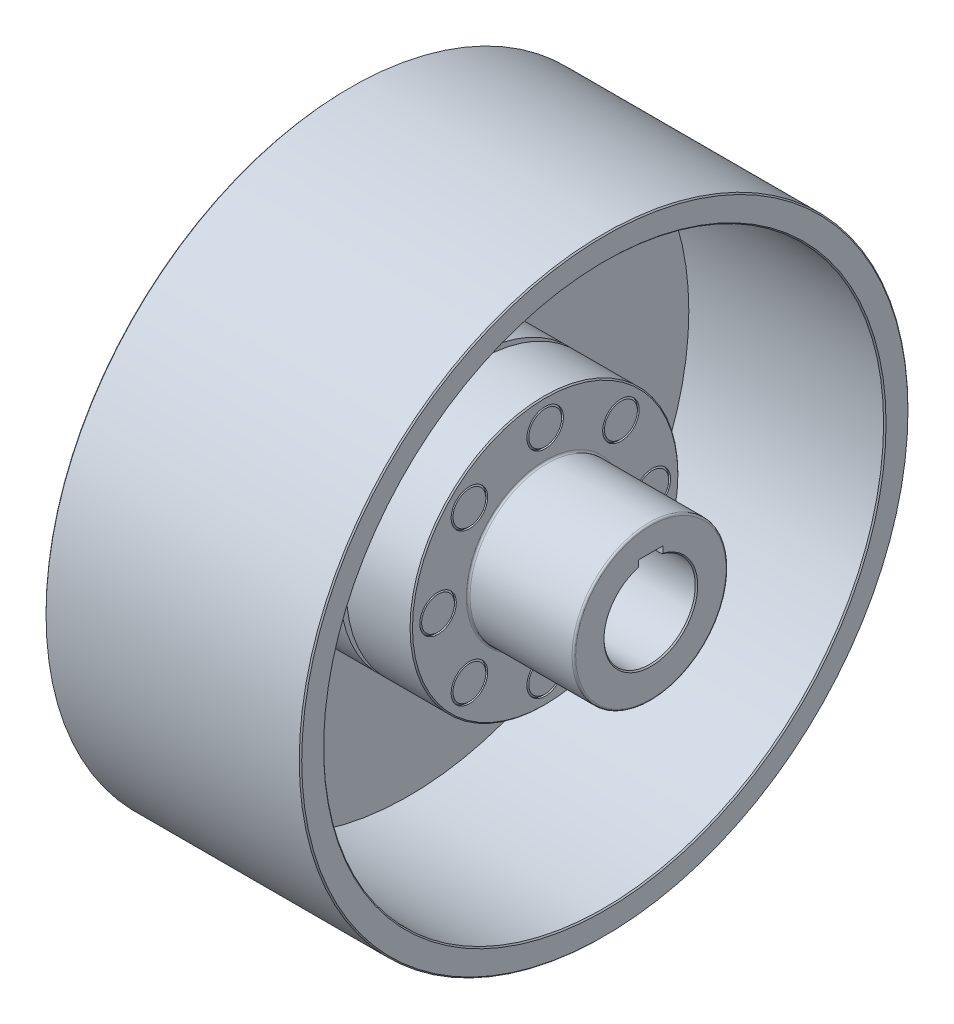
from build123d import *

# Parameters (mm, degrees)
CHAMFER1_SIZE      = 1
CHAMFER2_SIZE      = 1
CHAMFER3_SIZE      = 1
FILLET1_R          = 1.5
FILLET2_R          = 1.5
EXTRUDE1_DEPTH     = 3.375
CIRPATTERN11_COUNT = 8
SKETCH6_W          = 20
SKETCH6_H          = 9.8
CUT_EXTRUDE1_DEPTH = 455.496820734


with BuildPart() as part:
    # Sketch1 → Revolve1 (revolve)
    with BuildSketch(Plane.XY, mode=Mode.PRIVATE) as revolve1_sk:
        Polygon((-2.8, 56.925), (-30.8, 56.925), (-30.8, 37.5), (-142.8, 37.5), (-142.8, 63.25), (-61.6, 63.25), (-61.6, 68.85), (-56, 68.85), (-56, 110), (-2.8, 110), (-2.8, 104.5), (2.8, 104.5), (2.8, 110), (56, 110), (56, 63.25), (142.8, 63.25), (142.8, 37.5), (2.8, 37.5), (2.8, 0), (-2.8, 0), align=None)
    revolve(revolve1_sk.sketch.rotate(Axis((-114.849033811, 0, 0), (1, 0, 0)), 90), axis=Axis((-114.849033811, 0, 0), (1, 0, 0)))

    # Sketch2 → Revolve2 (revolve)
    with BuildSketch(Plane.XY, mode=Mode.PRIVATE) as revolve2_sk:
        Polygon((105, 250), (-105, 250), (-105, 230), (-61.6, 230), (-61.6, 68.85), (-56, 68.85), (-56, 230), (105, 230), align=None)
    revolve(revolve2_sk.sketch.rotate(Axis((0, 0, 0), (-1, 0, 0)), 90), axis=Axis((0, 0, 0), (-1, 0, 0)))

    # Sketch3 → Cut-Revolve1 (revolve, cut)
    with BuildSketch(Plane.XY, mode=Mode.PRIVATE) as cut_revolve1_sk:
        Polygon((-56, 103), (-61.6, 103), (-61.6, 88), (-56, 88), (-56, 101.5), (-54.5, 103), align=None)
        Polygon((56, 103), (54.5, 103), (56, 101.5), align=None)
    cut_revolve1 = revolve(cut_revolve1_sk.sketch.rotate(Axis((-61.6, 88, 0), (1, 0, 0)), 180), axis=Axis((-61.6, 88, 0), (1, 0, 0)), mode=Mode.SUBTRACT)

    # Chamfer1
    chamfer1_edges = [part.edges().sort_by_distance(p)[0] for p in [
        (142.8, 0, -37.5),
        (56, 0, -110),
    ]]
    chamfer(chamfer1_edges, length=CHAMFER1_SIZE)

    # Chamfer2
    chamfer2_edges = [part.edges().sort_by_distance(p)[0] for p in [
        (105, 0, 250),
        (105, 0, 230),
        (-105, 0, 230),
        (-105, 0, 250),
    ]]
    chamfer(chamfer2_edges, length=CHAMFER2_SIZE)

    # Chamfer3
    chamfer3_edges = [part.edges().sort_by_distance(p)[0] for p in [
        (-142.8, 0, -37.5),
    ]]
    chamfer(chamfer3_edges, length=CHAMFER3_SIZE)

    # Fillet1
    fillet1_edges = [part.edges().sort_by_distance(p)[0] for p in [
        (-61.6, 0, -63.25),
        (-142.8, 0, -63.25),
    ]]
    fillet(fillet1_edges, radius=FILLET1_R)

    # Fillet2
    fillet2_edges = [part.edges().sort_by_distance(p)[0] for p in [
        (142.8, 0, -63.25),
        (56, 0, -63.25),
    ]]
    fillet(fillet2_edges, radius=FILLET2_R)

    # Sketch5 → Extrude1 (add)
    with BuildSketch(Plane.ZY.offset(61.6)):
        Polygon((33.676142048, 76.971271842), (37.426142048, 79.136335352), (37.426142048, 83.46646237), (33.676142048, 85.63152588), (29.926142048, 83.46646237), (29.926142048, 79.136335352), align=None)
    extrude1 = extrude(amount=EXTRUDE1_DEPTH)

    # CirPattern11: Cut-Revolve1, Extrude1 ×8 about axis
    cirpattern11_axis = Axis((0, 0, 0), (1, 0, 0))
    add([cut_revolve1.rotate(cirpattern11_axis, i * 360 / CIRPATTERN11_COUNT) for i in range(1, CIRPATTERN11_COUNT)], mode=Mode.SUBTRACT)
    add([extrude1.rotate(cirpattern11_axis, i * 360 / CIRPATTERN11_COUNT) for i in range(1, CIRPATTERN11_COUNT)])

    # Sketch6 → Cut-Extrude1 (cut, through all)
    with BuildSketch(Plane(origin=(142.8, 0, 0), x_dir=(0, 0, -1), z_dir=(1, 0, 0))):
        with Locations((0, 37.5)):
            Rectangle(SKETCH6_W, SKETCH6_H)
    extrude(amount=-CUT_EXTRUDE1_DEPTH, mode=Mode.SUBTRACT)


solid = part.part
